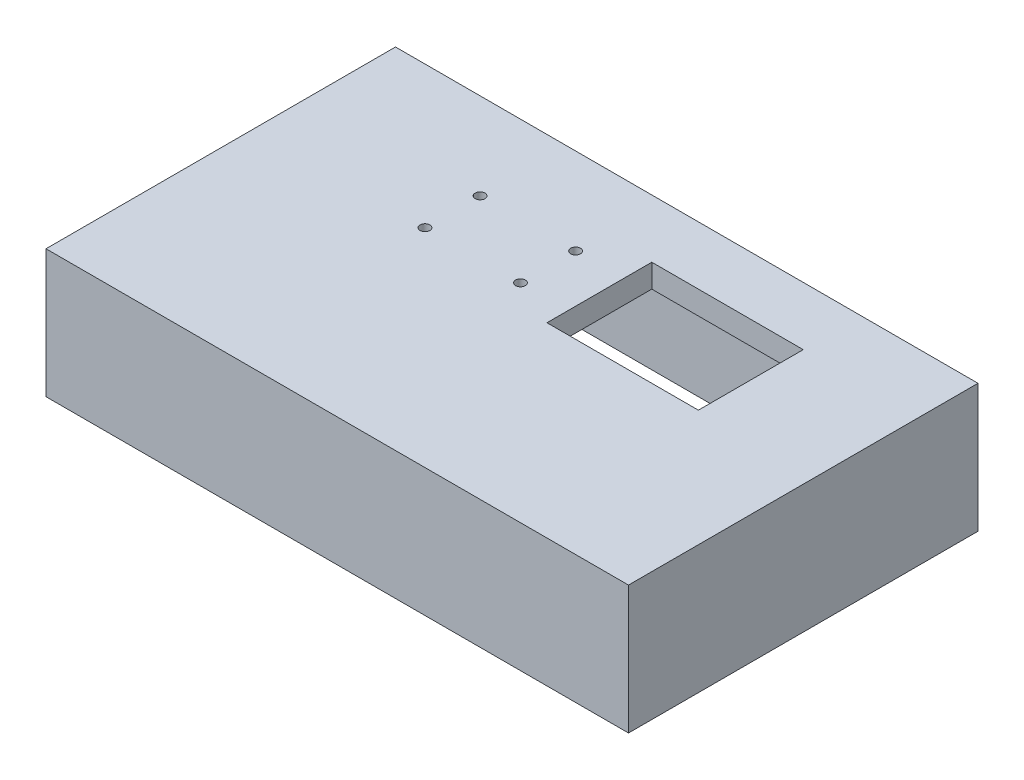
from build123d import *

# Parameters (mm, degrees)
SKETCH_1_W          = 250
SKETCH_1_H          = 55
EXTRUDE_1_DEPTH     = 150
SKETCH_2_W          = 230
SKETCH_2_H          = 130
CUT_EXTRUDE_1_DEPTH = 45
SKETCH_4_W          = 65
SKETCH_4_H          = 45
CUT_EXTRUDE_2_DEPTH = 223.093390385
SKETCH_10_R         = 2.1
CUT_EXTRUDE_8_DEPTH = 17.7


with BuildPart() as part:
    # 草图1 → 凸台-拉伸1 (new body)
    with BuildSketch(Plane.XY):
        with Locations((-32.481662592, 40.947432763)):
            Rectangle(SKETCH_1_W, SKETCH_1_H)
    extrude(amount=EXTRUDE_1_DEPTH)

    # 草图2 → 切除-拉伸1 (cut)
    with BuildSketch(Plane.XZ.offset(-13.447432763)):
        with Locations((-32.481662592, 75)):
            Rectangle(SKETCH_2_W, SKETCH_2_H)
    extrude(amount=-CUT_EXTRUDE_1_DEPTH, mode=Mode.SUBTRACT)

    # 草图4 → 切除-拉伸2 (cut, through all)
    with BuildSketch(Plane.XZ.offset(-58.447432763)):
        with Locations((10.018337408, 47.5)):
            Rectangle(SKETCH_4_W, SKETCH_4_H)
    extrude(amount=-CUT_EXTRUDE_2_DEPTH, mode=Mode.SUBTRACT)

    # 草图10 → 切除-拉伸8 (cut)
    with BuildSketch(Plane(origin=(971.262341276, 76.147432763, 1019.143932915), x_dir=(1, 0, 0), z_dir=(0, 1, 0))):
        with Locations(Location((-1055.250263055, 981.942263912, 0), (0, 0, 270))):
            Circle(SKETCH_10_R)
        with Locations(Location((-1055.250263055, 958.292263912, 0), (0, 0, 270))):
            Circle(SKETCH_10_R)
        with Locations(Location((-1014.250263055, 958.292263912, 0), (0, 0, 270))):
            Circle(SKETCH_10_R)
        with Locations(Location((-1014.250263055, 981.942263912, 0), (0, 0, 270))):
            Circle(SKETCH_10_R)
    extrude(amount=-CUT_EXTRUDE_8_DEPTH, mode=Mode.SUBTRACT)


solid = part.part
